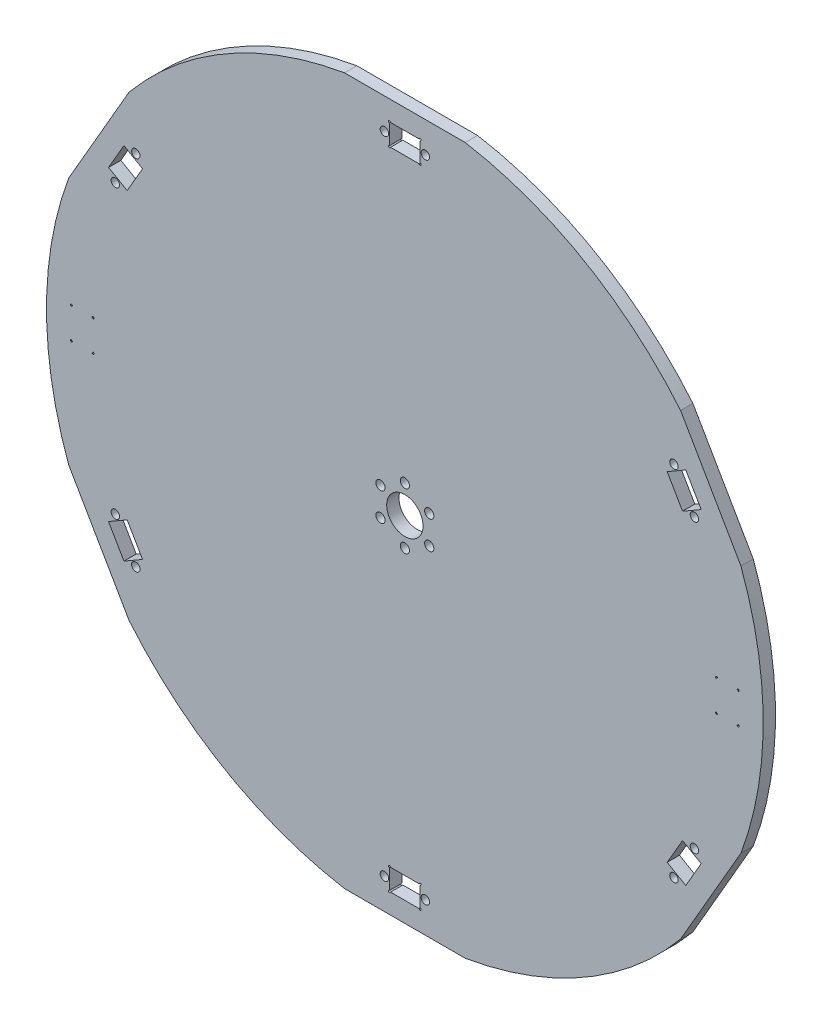
SolidWorks part; units mm, degrees
material "1023 碳钢板 (SS)"
ref_plane "前视基准面" through (0, 0, 0) normal (0, 0, 1) x (1, 0, 0)
ref_plane "上视基准面" through (0, 0, 0) normal (0, 1, 0) x (1, 0, 0)
ref_plane "右视基准面" through (0, 0, 0) normal (1, 0, 0) x (0, 0, -1)
sketch "草图1" plane through (0, 0, 0) normal (0, 0, 1) x (1, 0, 0)
  circle A0 centre (0, 0) radius 350
  circle A1 centre (0, 0) radius 17.75
  dimension "D1" = 700
  dimension "D2" = 35.5
extrude "凸台-拉伸1" add sketch "草图1" along normal mid plane 12 contours A1 | A0
sketch "草图2" plane through (0, 0, 6) normal (0, 0, 1) x (1, 0, 0)
  line L0 (0, -345) -> (0, 0) construction
  line L1 (58.9491, -355) -> (-58.9491, -355)
  line L2 (58.9491, -355) -> (58.9491, -345)
  line L3 (58.9491, -345) -> (-58.9491, -345)
  line L4 (-58.9491, -355) -> (-58.9491, -345)
  line L5 (58.9491, -355) -> (-58.9491, -345) construction
  line L6 (58.9491, -345) -> (-58.9491, -355) construction
  circle A0 centre (0, 0) radius 350 construction
  point P0 (0, -350)
  dimension "D1" = 345
extrude "切除-拉伸1" cut sketch "草图2" against normal up to next
pattern_circular "阵列(圆周)1" count 6 over 360 about axis through (0, 0, 0) along (0, 0, 1) of "切除-拉伸1"
sketch "草图3" plane through (0, 0, 6) normal (0, 0, 1) x (1, 0, 0)
  line L0 (0, -345) -> (0, -315) construction
  line L1 (15, -325.5) -> (-15, -325.5)
  line L2 (15, -325.5) -> (15, -304.5)
  line L3 (15, -304.5) -> (-15, -304.5)
  line L4 (-15, -325.5) -> (-15, -304.5)
  line L5 (15, -325.5) -> (-15, -304.5) construction
  line L6 (15, -304.5) -> (-15, -325.5) construction
  line L7 (58.9491, -345) -> (-58.9491, -345) construction
  point P0 (0, -315)
  dimension "D1" = 21
  dimension "D2" = 30
  dimension "D3" = 30
extrude "切除-拉伸2" cut sketch "草图3" against normal up to next
pattern_circular "阵列(圆周)2" count 6 over 360 about axis through (0, 0, 0) along (0, 0, 1) of "切除-拉伸2"
hole_wizard "M8 间隙孔1" positions "草图9" profile "草图10" hole size "M8" standard "GB" end condition up to next
sketch "草图9" plane through (0, 0, 6) normal (0, 0, 1) x (1, 0, 0)
  point P0 (-23.8157, -13.75)
sketch "草图10" plane through (-23.8157, -13.75, 6) normal (1, 0, 0) x (0, -1, 0)
  line L0 (0, 0) -> (0, 12)
  line L1 (0, 12) -> (4.5, 12)
  line L2 (4.5, 12) -> (4.5, 0)
  line L5 (4.5, 0) -> (0, 0)
  line L11 (0, -6.35) -> (0, 107.95) construction
  dimension "通孔孔直径" = 9
  dimension "通孔孔深度" = 12
pattern_circular "阵列(圆周)3" count 6 over 360 about axis through (0, 0, 0) along (0, 0, 1) of "M8 间隙孔1"
hole_wizard "Ø8.2 (8.2) 直径孔1" positions "草图13" profile "草图14" hole size "Ø8.2" standard "GB"
sketch "草图13" plane through (0, 0, 6) normal (0, 0, 1) x (1, 0, 0)
  line L0 (-20, -315) -> (0, -315) construction
  line L1 (0, -315) -> (0, -325.5) construction
  line L2 (-15, -325.5) -> (15, -325.5) construction
  line L5 (0, -315) -> (15, -315) construction
  line L6 (15, -325.5) -> (15, -304.5) construction
  point P0 (-20, -315)
  point P2 (20, -315)
  dimension "D1" = 20
sketch "草图14" plane through (-20, -315, 6) normal (1, 0, 0) x (0, -1, 0)
  line L0 (0, 0) -> (0, 10.4635)
  line L1 (0, 10.4635) -> (4.1, 8)
  line L2 (4.1, 8) -> (4.1, 0)
  line L5 (4.1, 0) -> (0, 0)
  line L10 (0, 10.4635) -> (-4.1, 8) construction
  line L11 (0, -6.35) -> (0, 107.95) construction
  dimension "孔直径" = 8.2
  dimension "孔深度" = 8
  dimension "导头角度" = 118
pattern_circular "阵列(圆周)5" count 6 over 360 about axis through (0, 0, 0) along (0, 0, 1) of "Ø8.2 (8.2) 直径孔1"
sketch "草图15" plane through (0, 0, 6) normal (0, 0, 1) x (1, 0, 0)
  circle A0 centre (-15, -325.5) radius 1
  circle A1 centre (15, -325.5) radius 1
  circle A2 centre (-15, -304.5) radius 1
  circle A3 centre (15, -304.5) radius 1
  dimension "D1" = 2
extrude "切除-拉伸3" cut sketch "草图15" against normal up to next
pattern_circular "阵列(圆周)6" count 4 over 360 about axis through (0, 0, 0) along (0, 0, 1) of "切除-拉伸3"
